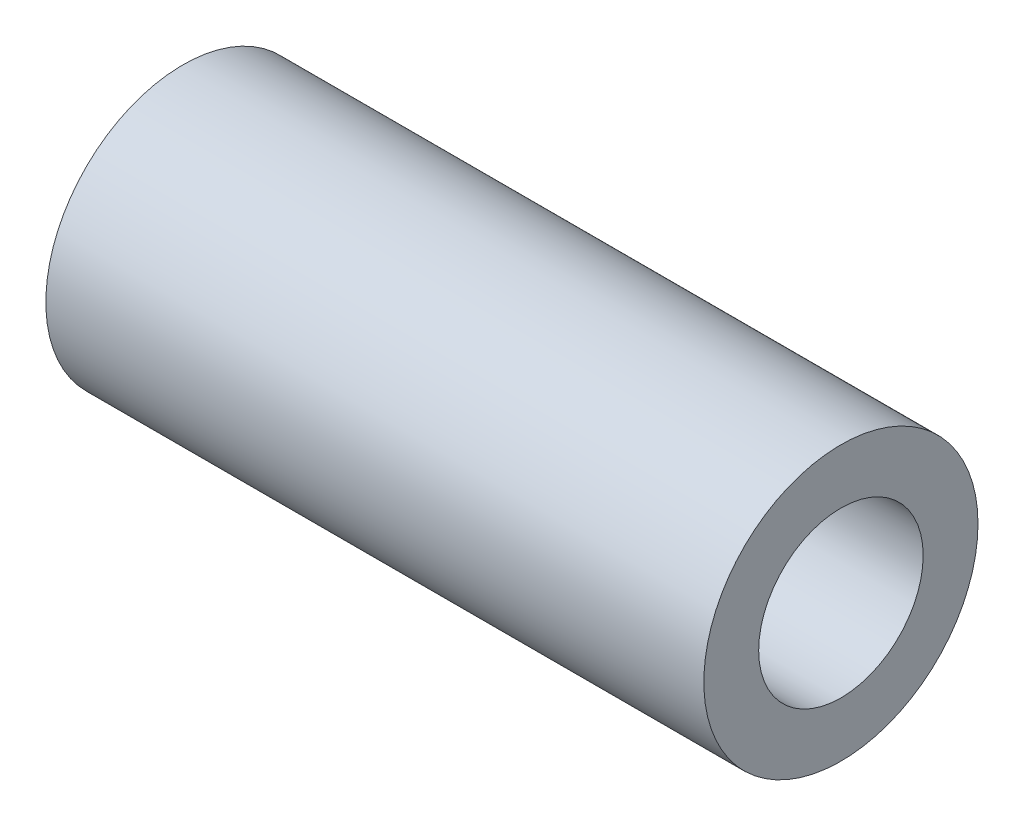
from build123d import *

# Parameters (mm, degrees)
SKETCH_1_R      = 2.5
SKETCH_1_R_2    = 1.5
EXTRUDE_1_DEPTH = 12


with BuildPart() as part:
    # 草图1 → 凸台-拉伸1 (new body)
    with BuildSketch(Plane(origin=(0, 0, 0), x_dir=(0, 0, -1), z_dir=(1, 0, 0))):
        Circle(SKETCH_1_R)
        Circle(SKETCH_1_R_2, mode=Mode.SUBTRACT)
    extrude(amount=EXTRUDE_1_DEPTH)


solid = part.part
